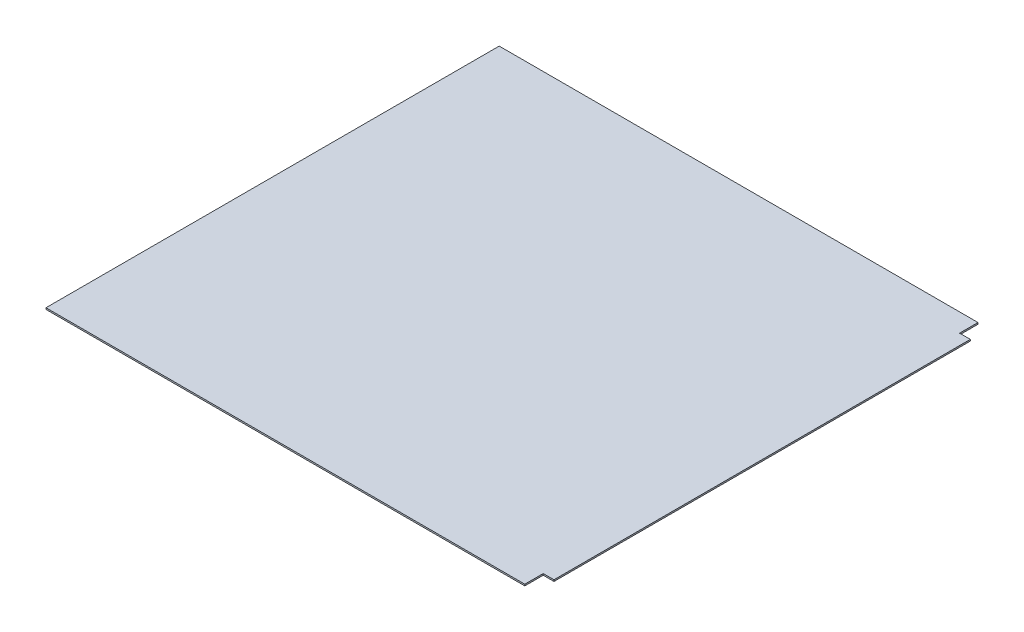
from build123d import *

# Parameters (mm, degrees)
BOSS_EXTRUDE1_DEPTH = 3


with BuildPart() as part:
    # Sketch1 → Boss-Extrude1 (new body)
    with BuildSketch(Plane(origin=(0, 0, 0), x_dir=(1, 0, 0), z_dir=(0, 1, 0))):
        Polygon((-21, -406.5), (0, -406.5), (0, 406.5), (-21, 406.5), (-21, 442.5), (-956, 442.5), (-956, -442.5), (-21, -442.5), align=None)
    extrude(amount=BOSS_EXTRUDE1_DEPTH)


solid = part.part
